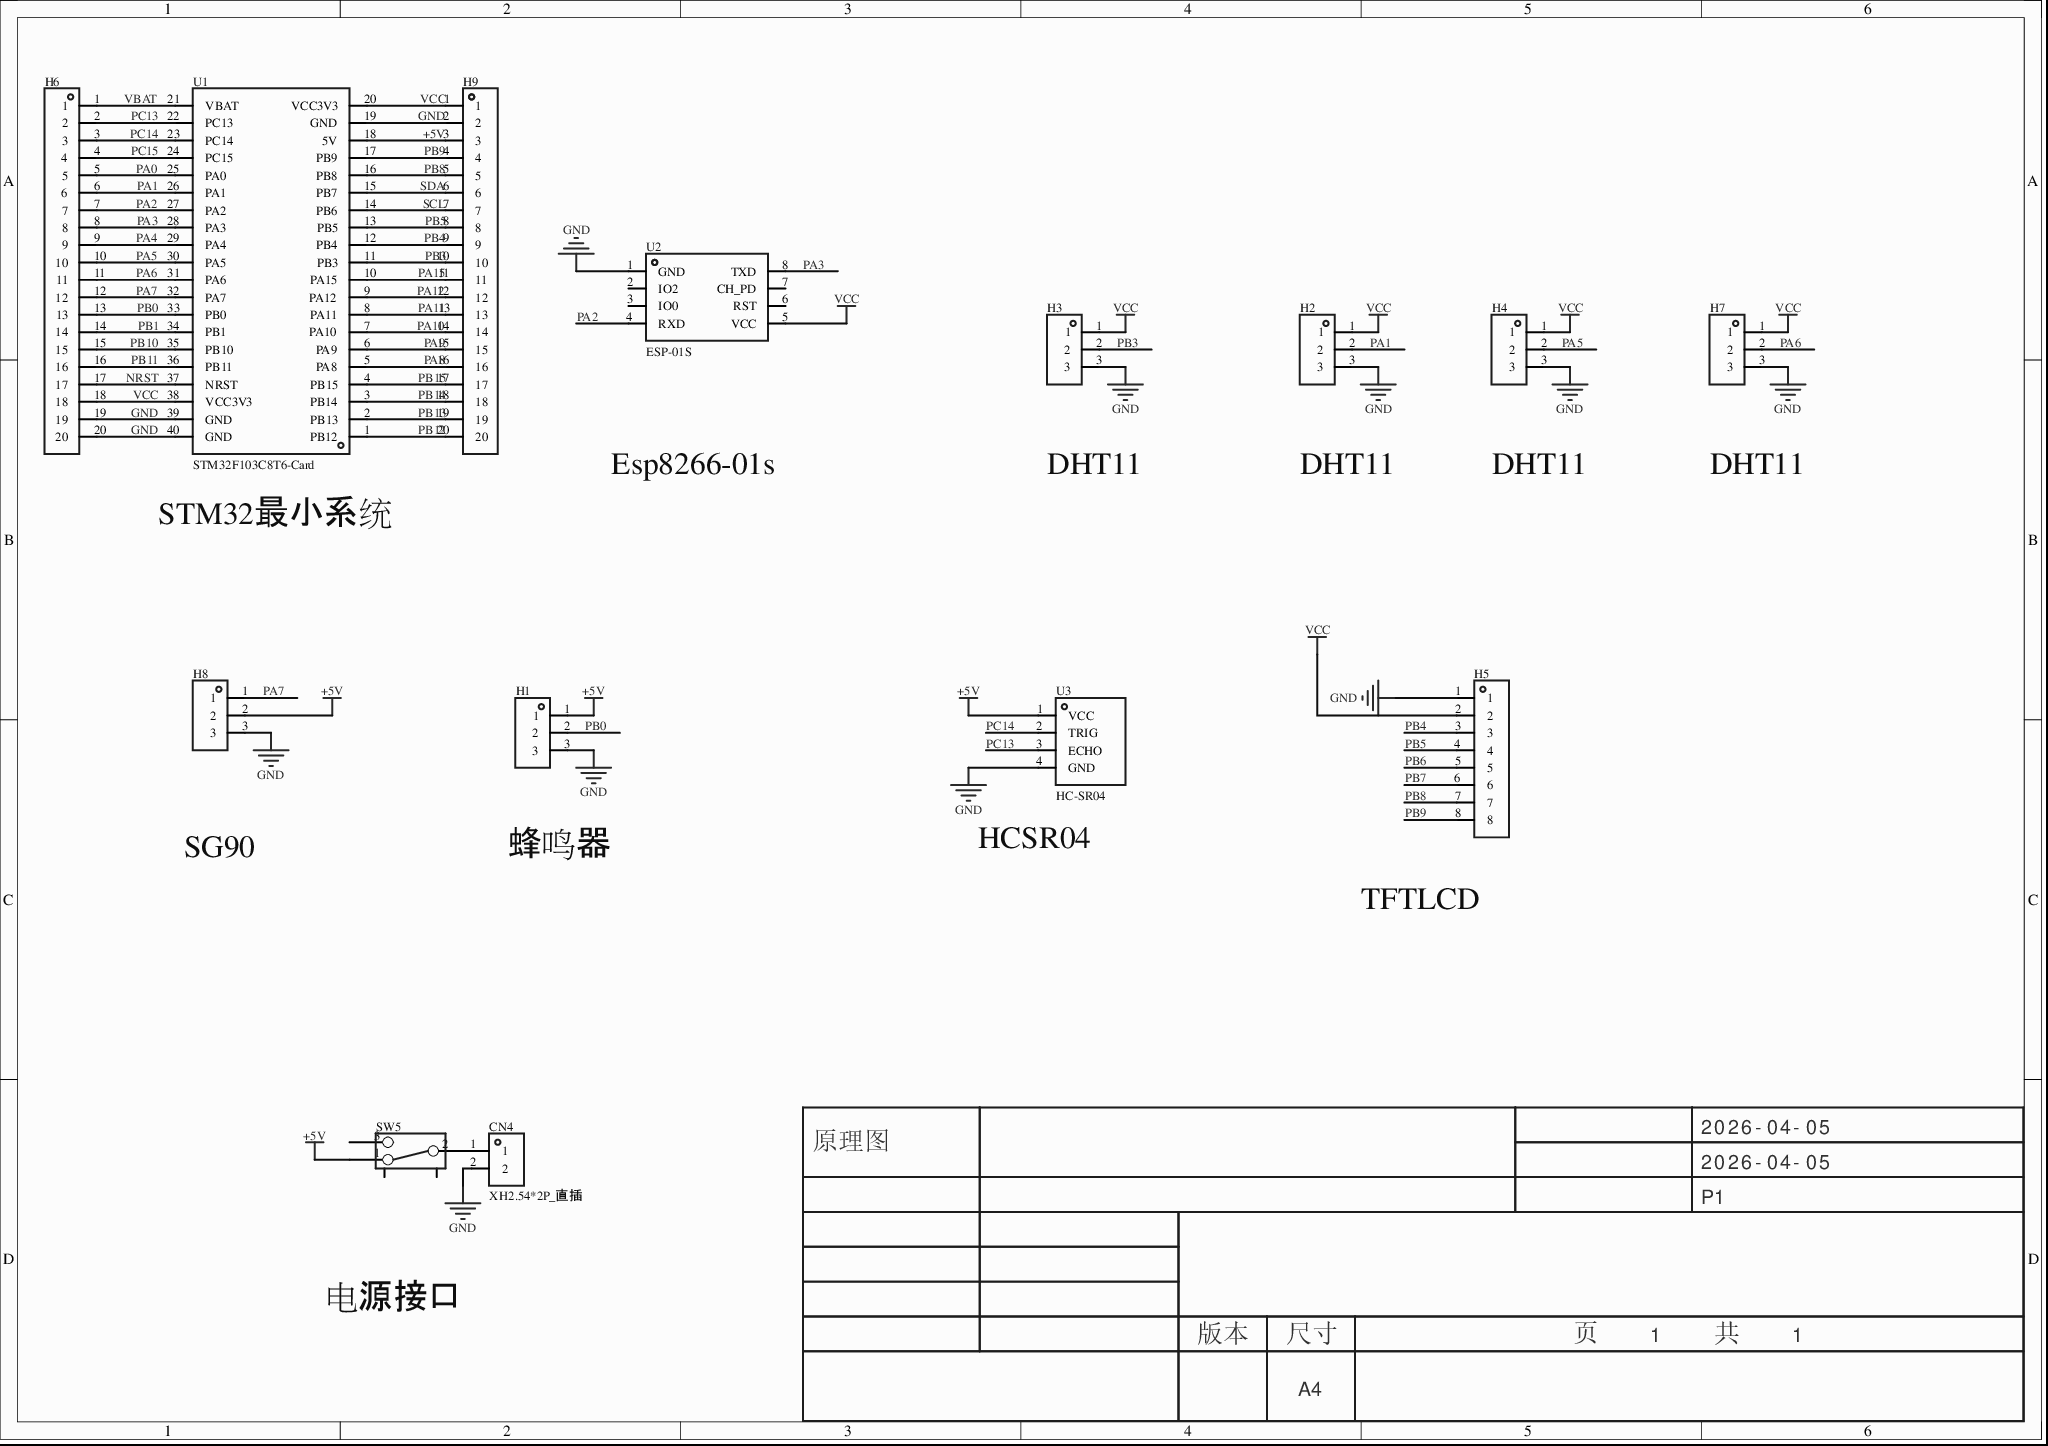
[diagram p0: MISC50977-3.schdoc]
# Altium project MISC50977-2.PrjPcb
1 sheet, 14 parts. Net scope: global (net labels, ports and power ports of the same name join across sheets).
Board file: MISC50977.pcbdoc

## Sheet MISC50977-3.schdoc
size 297 x 209 mm; Version: V1.0; @Project Name: MISC50977; @Update Date: 2026-04-05; @Create Date: 2026-04-05; @Board Name: MISC50977; @Create Time: 23:41:37; @Page Count: 1; @Page No: 1; @Schematic Name: MISC50977; @Update Time: 23:41:37; Size: A4

### Parts
CN4  XH2.54*2P_直插  [CONN-TH_2P-P2.50-XH2.54-2P]
H1  (no value)  [HDR-TH_3P-P2.54-V-F]
H2  (no value)  [HDR-TH_3P-P2.54-V-F]
H3  (no value)  [HDR-TH_3P-P2.54-V-F]
H4  (no value)  [HDR-TH_3P-P2.54-V-F]
H5  (no value)  [HDR-TH_8P-P2.54-V-F-1]
H6  (no value)  [HDR-TH_20P-P2.54-V-M-1]
H7  (no value)  [HDR-TH_3P-P2.54-V-F]
H8  (no value)  [HDR-TH_3P-P2.54-V-F]
H9  (no value)  [HDR-TH_20P-P2.54-V-M-1]
SW5  (no value)  [拨动开关]
U1  STM32F103C8T6-Card  [CONN-TH_L53.3-W22.9_STM32F103C8T6-CARD]
U2  ESP-01S  [WIFIM-TH_ESP-01S]
U3  HC-SR04  [TH_HC-SR04V]

### Nets
+5V: H1.1 H8.2 H9.3 SW5.1 U1.18(5V) U3.1(VCC)
GND: CN4.2 H1.3 H2.3 H3.3 H4.3 H5.1 H6.19 H6.20 H7.3 H8.3 H9.2 U1.19(GND) U1.39(GND) U1.40(GND) U2.1(GND) U3.4(GND)
VCC: H2.1 H3.1 H4.1 H5.2 H6.18 H7.1 H9.1 U1.20(VCC3V3) U1.38(VCC3V3) U2.5(VCC)
NRST: H6.17 U1.37(NRST)
PA0: H6.5 U1.25(PA0)
PA1: H2.2 H6.6 U1.26(PA1)
PA2: H6.7 U1.27(PA2) U2.4(RXD)
PA3: H6.8 U1.28(PA3) U2.8(TXD)
PA4: H6.9 U1.29(PA4)
PA5: H4.2 H6.10 U1.30(PA5)
PA6: H6.11 H7.2 U1.31(PA6)
PA7: H6.12 H8.1 U1.32(PA7)
PA8: H9.16 U1.5(PA8)
PA9: H9.15 U1.6(PA9)
PA10: H9.14 U1.7(PA10)
PA11: H9.13 U1.8(PA11)
PA12: H9.12 U1.9(PA12)
PA15: H9.11 U1.10(PA15)
PB0: H1.2 H6.13 U1.33(PB0)
PB1: H6.14 U1.34(PB1)
PB3: H3.2 H9.10 U1.11(PB3)
PB4: H5.3 H9.9 U1.12(PB4)
PB5: H5.4 H9.8 U1.13(PB5)
PB6: H5.5
PB7: H5.6
PB8: H5.7 H9.5 U1.16(PB8)
PB9: H5.8 H9.4 U1.17(PB9)
PB10: H6.15 U1.35(PB10)
PB11: H6.16 U1.36(PB11)
PB12: H9.20 U1.1(PB12)
PB13: H9.19 U1.2(PB13)
PB14: H9.18 U1.3(PB14)
PB15: H9.17 U1.4(PB15)
PC13: H6.2 U1.22(PC13) U3.3(ECHO)
PC14: H6.3 U1.23(PC14) U3.2(TRIG)
PC15: H6.4 U1.24(PC15)
SCL: H9.7 U1.14(PB6)
SDA: H9.6 U1.15(PB7)
VBAT: H6.1 U1.21(VBAT)
NetCN4_1: CN4.1 SW5.2

Not connected (* = marked no-connect by the designer): SW5 3 4 5; U2 2(IO2)* 3(IO0)* 6(RST)* 7(CH_PD)*

### Notes on the sheet
- Esp8266-01s
- DHT11
- (near U1) STM32最小系统
- SG90
- 蜂鸣器
- (near U3) HCSR04
- (near H5) TFTLCD
- 电源接口
- 2026-04-05
- 原理图
- P1
- 版本
- 尺寸
- A4
- 页    1    共    1

### Library data of the parts
CN4 = XH2.54*2P_直插: 3D Model: 325c595e30db4df8abe76612dd40b0fa0819f05c4eef4c71ace90d822a990e87; 3D Model Transform: 295.275,228.346,0,180,0,0,-0.002,-20.079,-137.795; AddInBom: yes; Symbol: XH2.54*2P_直插; Device: XH2.54*2P_直插; LCSC Part Name: XH2.54*2P_直插; Supplier Part: C9900008615; Manufacturer Part: XH2.54*2P_直插; Supplier Footprint: XH2.54_2P; JLCPCB Part Class: Extended Part; Supplier: LCSC; ConvertToPcb: yes; FootprintName: CONN-TH_2P-P2.50-XH2.54-2P; ModelName: CONN-TH_2P-P2.50-XH2.54-2P
H1-H4 H7 H8 = HDR-F_2.54_1x3P: Symbol: PM254V-11-03-H85; 3D Model: f3b3cc5aae9641bf9e56fc160cef875b; 3D Model Transform: 299.9994,100,0,0,0,0,0,0,-118.11; ConvertToPcb: yes; ModelName: HDR2.54-F-LI-1X3P; Device: HDR-F_2.54_1x3P; Supplier Part: C541850; Supplier Footprint: 插件; AddInBom: yes; FootprintName: HDR-TH_3P-P2.54-V-F
H5 = HDR-F_2.54_1x8P: Symbol: Header-Female-2.54_1x8; AddInBom: yes; ModelId: 0f7e4d9227ef4fa08d5469c22cc70cdb0819f05c4eef4c71ace90d822a990e87; ModelName: HDR-F-2.54_1x8; ModelTransform: 799.99844,100,0,0,0,0,0,0,-118.11; Device: HDR-F_2.54_1x8P; ConvertToPcb: yes; FootprintName: HDR-TH_8P-P2.54-V-F-1; SupplierPart: C27438; Supplier Footprint: 插件
H6 H9 = HDR-M_2.54_1x20P: 间距:2.54mm;总PIN位数:20;排数:1;插针结构:-;行距:-;安装类型:直插;圆针/方针:-;额定电流:-;额定电压:-;配合针长度:-;塑高:-;触头材质:黄铜;触头镀层:-;颜色:黑色;; Symbol: HDR_2.54-1x20P; ConvertToPcb: yes; ModelId: f68709be121d406db68b06f32a5953890819f05c4eef4c71ace90d822a990e87; ModelName: HDR-M-2.54_1x20; ModelTransform: 1999.996,100,0,0,0,0,0,0,-118.11; Device: HDR-M_2.54_1x20P; AddInBom: yes; SupplierPart: C50981; Supplier Footprint: 插件; FootprintName: HDR-TH_20P-P2.54-V-M-1
SW5 = 拨动开关_正: 3D Model: 4321fe59a4074cbfb4989553f297c68f0819f05c4eef4c71ace90d822a990e87; 3D Model Transform: 370.09,208.7,472.35,0,0,0,0,0,-110; ConvertToPcb: yes; ModelName: SW-TH_SS-12D02-VG4; Symbol: 拨动开关; Device: 拨动开关_正; Supplier Footprint: 插件; AddInBom: yes; FootprintName: 拨动开关
U1 = STM32F103C8T6-Card: AddInBom: yes; Symbol: STM32F103C8T6-CARD; Device: STM32F103C8T6-Card; LCSC Part Name: STM32F103C8T6-Card; Supplier Part: C9900077949; Manufacturer Part: STM32F103C8T6-Card; Supplier Footprint: 插件; Supplier: LCSC; ConvertToPcb: yes; FootprintName: CONN-TH_L53.3-W22.9_STM32F103C8T6-CARD
U2 = ESP-01S_C111009: 3D Model: eb7175da78ae48b3b1568cfe3027405f0819f05c4eef4c71ace90d822a990e87; 3D Model Transform: 582.676,976.37608,0,0,0,0,0,388.346,-118.11; AddInBom: yes; Symbol: ESP-01S; Device: ESP-01S_C111009; LCSC Part Name: ESP-01S; Supplier Part: C111009; Manufacturer Part: ESP-01S; Supplier Footprint: -; JLCPCB Part Class: Extended Part; Supplier: LCSC; ConvertToPcb: yes; FootprintName: WIFIM-TH_ESP-01S; ModelName: WIFIM-TH_ESP-01S
U3 = HC-SR04: Manufacturer: Universal Microelectronics; AddInBom: yes; Symbol: HC-SR04; Device: HC-SR04; LCSC Part Name: HC-SR04; SupplierPart: C19857336; ManufacturerPart: HC-SR04; Supplier Footprint: -; JLCPCB Part Class: Extended Part; Datasheet: https://item.szlcsc.com/datasheet/HC-SR04/21184790.html; Supplier: LCSC; ConvertToPcb: yes; FootprintName: TH_HC-SR04V